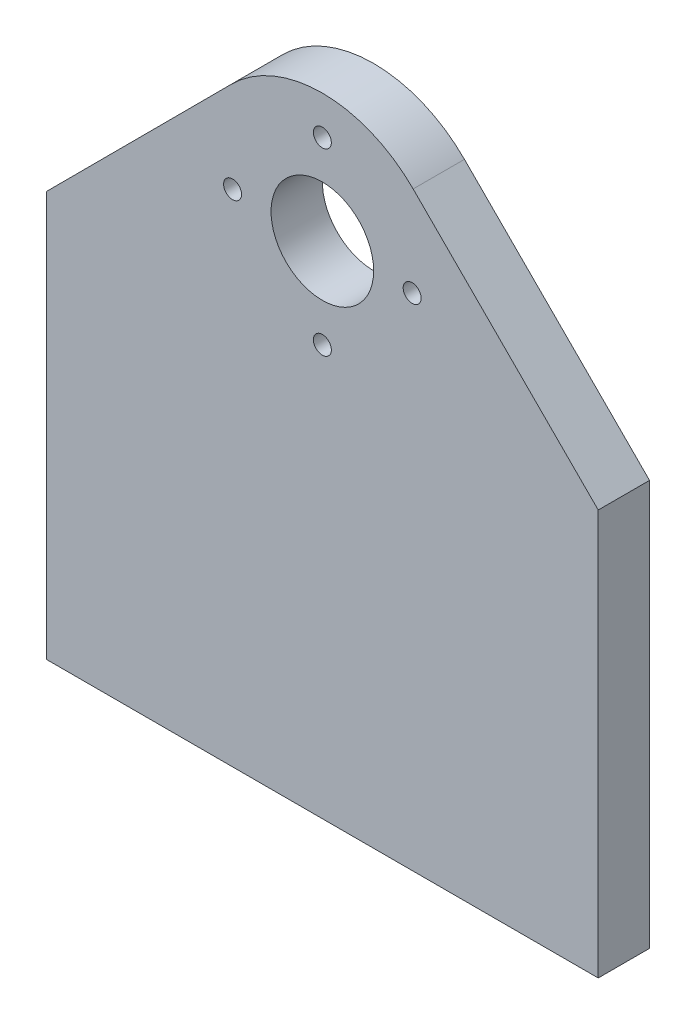
SolidWorks part; units mm, degrees
ref_plane "Front Plane" through (0, 0, 0) normal (0, 0, 1) x (1, 0, 0)
ref_plane "Top Plane" through (0, 0, 0) normal (0, 1, 0) x (1, 0, 0)
ref_plane "Right Plane" through (0, 0, 0) normal (1, 0, 0) x (0, 0, -1)
sketch "Sketch1" plane through (0, 0, 0) normal (0, 0, 1) x (1, 0, 0)
  line L0 (0, 0) -> (430.2, 0)
  line L1 (430.2, 0) -> (430.2, 316)
  line L2 (0, 0) -> (0, 316)
  line L3 (0, 316) -> (144.3107, 460.632)
  line L4 (430.2, 316) -> (285.8893, 460.632)
  arc A0 (285.8893, 460.632) -> (144.3107, 460.632) centre (215.1, 390) ccw
  circle A1 centre (215.1, 390) radius 40
  dimension "D6" = 200
  dimension "D7" = 80
  dimension "D1" = 430.2
  dimension "D2" = 316
  dimension "D3" = 316
  dimension "D4" = 390
  dimension "D5" = 215.1
extrude "Boss-Extrude1" add sketch "Sketch1" along normal blind 40
hole_wizard "M16 Tapped Hole1" positions "Sketch3" profile "Sketch2" tap size "M16" standard "GB" end condition through all
sketch "Sketch3" plane through (0, 0, 40) normal (0, 0, 1) x (1, 0, 0)
  circle A0 centre (215.1, 390) radius 70
  point P0 (215.1, 460)
  point P27 (285.1, 390)
  point P28 (215.1, 320)
  point P29 (145.1, 390)
  dimension "D1" = 140
  dimension "D2" = 4
sketch "Sketch2" plane through (215.1, 460, 40) normal (1, 0, 0) x (0, -1, 0)
  line L0 (0, 0) -> (0, 40)
  line L1 (0, 40) -> (7, 40)
  line L2 (7, 40) -> (7, 0)
  line L5 (7, 0) -> (0, 0)
  line L11 (0, -6.35) -> (0, 107.95) construction
  dimension "通孔螺纹孔钻头直径" = 14
  dimension "通孔螺纹孔钻头深度" = 40
cosmetic thread "CosmeticThread hole thread 1" parameters "D2"=16
cosmetic thread "CosmeticThread hole thread 2" parameters "D2"=16
cosmetic thread "CosmeticThread hole thread 3" parameters "D2"=16
cosmetic thread "CosmeticThread hole thread 4" parameters "D2"=16
